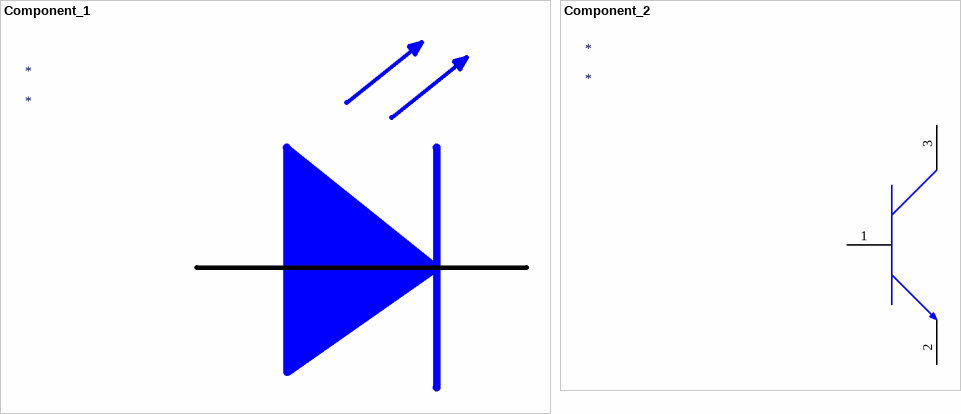
[diagram p0: symbols Component_1 to Component_2]
# Altium schematic symbol library MISC82341-27.SchLib: 2 symbols
Pins are listed as number, name and electrical type; pins without a type are passive.


## Component_1
designator *

## Component_2
designator *
pins: 1, 2, 3